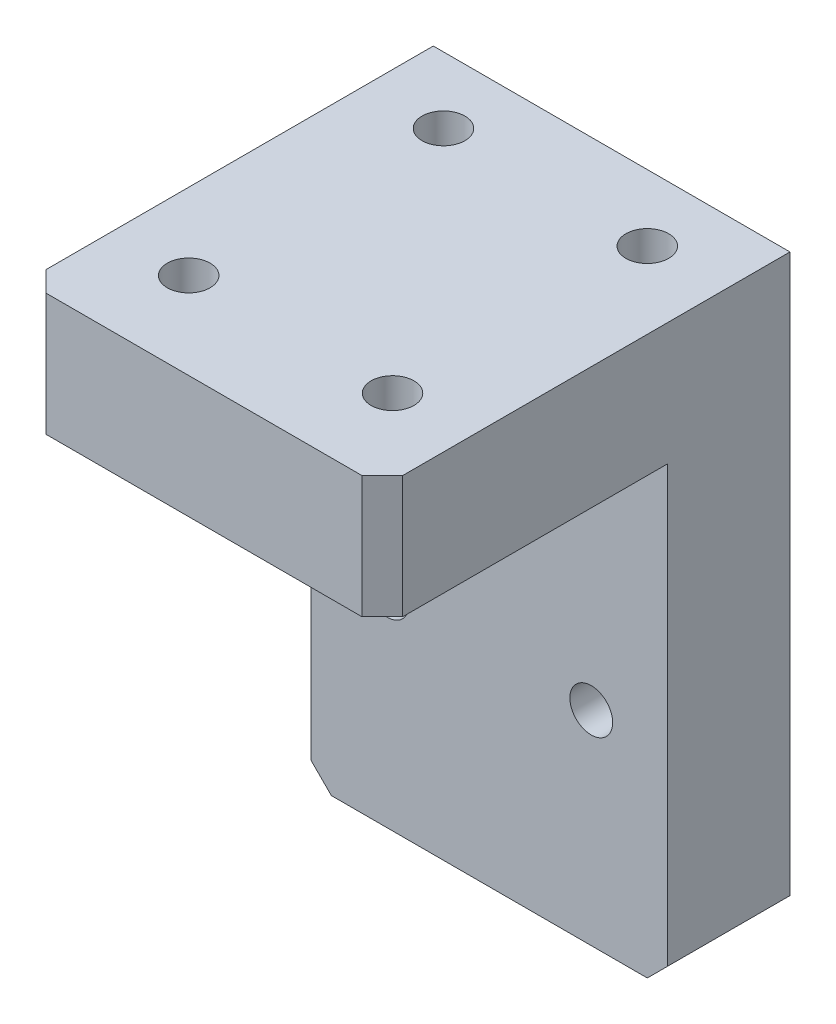
from build123d import *

# Parameters (mm, degrees)
SKETCH_1_W             = 35
SKETCH_1_H             = 56.7
EXTRUDE_1_DEPTH        = 12
CHAMFER_1_SIZE         = 2
SKETCH_4_W             = 28
SKETCH_4_H             = 12
EXTRUDE_2_DEPTH        = 35
HOLE_WIZARD_M5_1_D     = 4.2
CHAMFER_2_SIZE         = 2
HOLE_WIZARD_M5_2_D     = 4.2
HOLE_WIZARD_M5_2_DEPTH = 12.4
HOLE_WIZARD_M5_2_TIP   = 1.2618073


with BuildPart() as part:
    # 草图1 → 凸台-拉伸1 (new body)
    with BuildSketch(Plane.XY):
        Rectangle(SKETCH_1_W, SKETCH_1_H)
    extrude(amount=EXTRUDE_1_DEPTH)

    # 倒角1
    chamfer_1_edges = [part.edges().sort_by_distance(p)[0] for p in [
        (-17.5, -28.35, 6),
        (17.5, -28.35, 6),
    ]]
    chamfer(chamfer_1_edges, length=CHAMFER_1_SIZE)

    # 草图4 → 凸台-拉伸2 (add)
    with BuildSketch(Plane.ZY.offset(17.5)):
        with Locations((26, 22.35)):
            Rectangle(SKETCH_4_W, SKETCH_4_H)
    extrude(amount=-EXTRUDE_2_DEPTH)

    # M5 螺纹孔1 (through all)
    with Locations(Plane(origin=(0, 0, 0), x_dir=(-1, 0, 0), z_dir=(0, 0, -1))):
        with Locations((-10, -8.35), (10, -8.35)):
            Hole(HOLE_WIZARD_M5_1_D / 2)

    # 倒角2
    chamfer_2_edges = [part.edges().sort_by_distance(p)[0] for p in [
        (-17.5, 22.35, 40),
        (17.5, 22.35, 40),
    ]]
    chamfer(chamfer_2_edges, length=CHAMFER_2_SIZE)

    # M5 螺纹孔2
    with Locations(Plane(origin=(0, 28.35, 0), x_dir=(1, 0, 0), z_dir=(0, 1, 0))):
        with Locations((-10, -6.5), (10, -6.5), (-10, -31.5), (10, -31.5)):
            Hole(HOLE_WIZARD_M5_2_D / 2, depth=HOLE_WIZARD_M5_2_DEPTH)
            with Locations((0, 0, -(HOLE_WIZARD_M5_2_DEPTH + HOLE_WIZARD_M5_2_TIP / 2))):  # 118° drill point
                Cone(0, HOLE_WIZARD_M5_2_D / 2, HOLE_WIZARD_M5_2_TIP, mode=Mode.SUBTRACT)


solid = part.part
